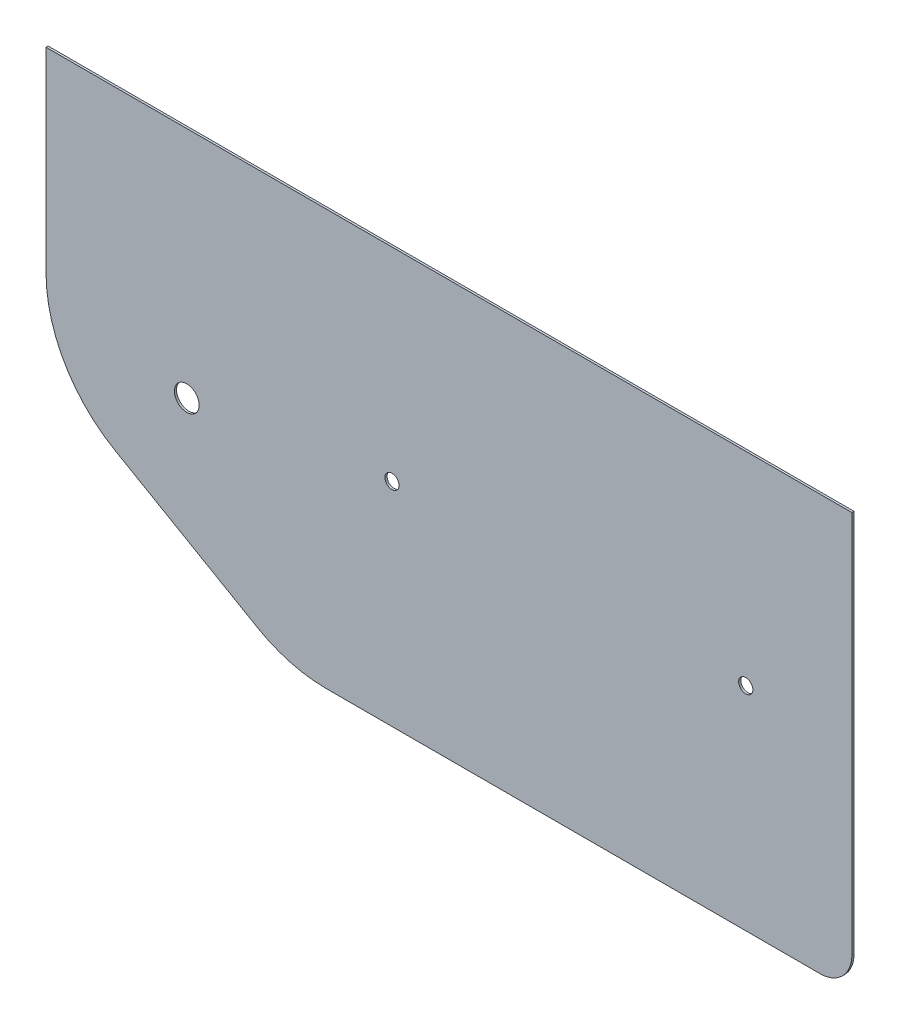
SolidWorks part; units mm, degrees
ref_plane "Front Plane" through (0, 0, 0) normal (0, 0, 1) x (1, 0, 0)
ref_plane "Top Plane" through (0, 0, 0) normal (0, 1, 0) x (1, 0, 0)
ref_plane "Right Plane" through (0, 0, 0) normal (1, 0, 0) x (0, 0, -1)
sketch "Sketch1" plane through (0, 0, 0) normal (0, 0, 1) x (1, 0, 0)
  line L0 (0, 587) -> (0, 45)
  line L1 (0, 587) -> (-1139, 587)
  line L2 (-1139, 587) -> (-1139, 311.1918)
  line L3 (-45, 0) -> (-742.7499, 0)
  line L4 (-840.2499, 26.125) -> (-1041.5, 142.3168)
  arc A0 (0, 45) -> (-45, 0) centre (-45, 45) cw
  arc A1 (-1139, 311.1918) -> (-1041.5, 142.3168) centre (-944, 311.1918) ccw
  arc A2 (-742.7499, 0) -> (-840.2499, 26.125) centre (-742.7499, 195) cw
  circle A3 centre (-650, 300) radius 10
  circle A4 centre (-150, 300) radius 10
  circle A5 centre (-940, 257) radius 17.5
  point P8 (0, 0)
  dimension "D2" = 45
  dimension "D3" = 195
  dimension "D1" = 150
extrude "Boss-Extrude1" add sketch "Sketch1" along normal blind 3
